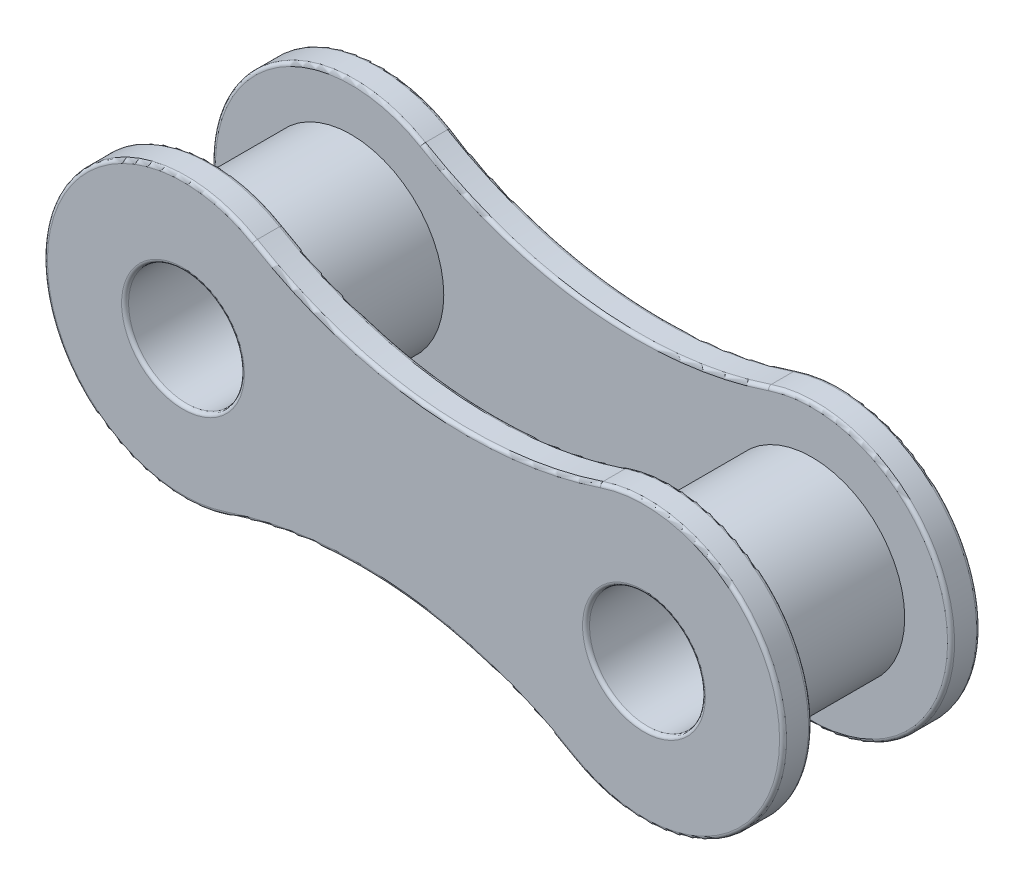
from build123d import *

# Parameters (mm, degrees)
BOSS_EXTRUDE1_DEPTH        = 3
BOSS_EXTRUDE1_DEPTH_BACK   = 3
SKETCH3_R                  = 4
SKETCH3_R_2                = 2.5
BOSS_EXTRUDE1_2_DEPTH      = 3
BOSS_EXTRUDE1_2_DEPTH_BACK = 3
SKETCH5_R                  = 2.5
BOSS_EXTRUDE2_DEPTH        = 1.25
FILLET1_R                  = 0.15
SCALE1_SCALE               = 0.5
SCALE2_SCALE               = 0.5
SCALE3_SCALE               = 0.5


with BuildPart() as part:
    # Sketch3 → Boss-Extrude1 (new, two sides: drawn at the far end of the back side and taken through both)
    with BuildSketch(Plane.XY.offset(-BOSS_EXTRUDE1_DEPTH_BACK)):
        with Locations((-87.399549733, 1.891684495)):
            Circle(SKETCH3_R)
        with Locations((-87.399549733, 1.891684495)):
            Circle(SKETCH3_R_2, mode=Mode.SUBTRACT)
    extrude(amount=BOSS_EXTRUDE1_DEPTH + BOSS_EXTRUDE1_DEPTH_BACK)


with BuildPart() as body_2:
    # Sketch3 → Boss-Extrude1 2 (new, two sides: drawn at the far end of the back side and taken through both)
    with BuildSketch(Plane.XY.offset(-BOSS_EXTRUDE1_2_DEPTH_BACK)):
        with Locations((-67.511724124, -0.223591499)):
            Circle(SKETCH3_R)
        with Locations((-67.511724124, -0.223591499)):
            Circle(SKETCH3_R_2, mode=Mode.SUBTRACT)
    extrude(amount=BOSS_EXTRUDE1_2_DEPTH + BOSS_EXTRUDE1_2_DEPTH_BACK)


with BuildPart() as body_3:
    # Sketch5 → Boss-Extrude2 (new body)
    with BuildSketch(Plane.XY.offset(3)):
        with BuildLine():
            ThreePointArc((-70.574575747, -5.382946104), (-61.545376441, -0.858174297), (-69.420828904, 5.464582104))
            ThreePointArc((-69.420828904, 5.464582104), (-77.051891637, 4.630059865), (-84.336698111, 7.0510391))
            ThreePointArc((-84.336698111, 7.0510391), (-93.365897416, 2.526267293), (-85.490444954, -3.796489108))
            ThreePointArc((-85.490444954, -3.796489108), (-77.85938222, -2.961966869), (-70.574575747, -5.382946104))
        make_face()
        with Locations((-67.511724124, -0.223591499)):
            Circle(SKETCH5_R, mode=Mode.SUBTRACT)
        with Locations((-87.399549733, 1.891684495)):
            Circle(SKETCH5_R, mode=Mode.SUBTRACT)
    extrude(amount=BOSS_EXTRUDE2_DEPTH)


with BuildPart() as body_4:
    # Mirror1: mirrored copy
    add(body_3.part.mirror(Plane.XY))


with BuildPart() as body_3_1:
    add(body_3.part)

    # Combine1: union part, body 4, body 2
    add(part.part)
    add(body_4.part)
    add(body_2.part)

    # Fillet1
    fillet1_edges = [body_3_1.edges().sort_by_distance(p)[0] for p in [
        (-70.011724124, -0.223591499, 4.25),
        (-77.051891637, 4.630059865, 4.25),
        (-89.899549733, 1.891684495, 4.25),
        (-93.365897416, 2.526267293, 4.25),
        (-70.011724124, -0.223591499, -4.25),
        (-89.899549733, 1.891684495, -4.25),
        (-77.85938222, -2.961966869, -3),
        (-61.545376441, -0.858174297, -3),
        (-77.051891637, 4.630059865, -3),
        (-93.365897416, 2.526267293, -3),
        (-77.85938222, -2.961966869, -4.25),
        (-61.545376441, -0.858174297, -4.25),
        (-77.051891637, 4.630059865, -4.25),
        (-93.365897416, 2.526267293, -4.25),
        (-77.85938222, -2.961966869, 4.25),
        (-93.365897416, 2.526267293, 3),
        (-77.051891637, 4.630059865, 3),
        (-61.545376441, -0.858174297, 3),
        (-77.85938222, -2.961966869, 3),
        (-61.545376441, -0.858174297, 4.25),
    ]]
    fillet(fillet1_edges, radius=FILLET1_R)


with BuildPart() as body_3_2:
    # Scale1: scaled about (-77.455636929, 0.834046498, 0)
    add(body_3_1.part.scale(SCALE1_SCALE).moved(Location((-38.727818464, 0.417023249, 0))))


with BuildPart() as body_3_3:
    # Scale2: scaled about (-77.455636929, 0.834046498, 0)
    add(body_3_2.part.scale(SCALE2_SCALE).moved(Location((-38.727818464, 0.417023249, 0))))


with BuildPart() as body_3_4:
    # Scale3: scaled about (-77.455636929, 0.834046498, 0)
    add(body_3_3.part.scale(SCALE3_SCALE).moved(Location((-38.727818464, 0.417023249, 0))))


solid = body_3_4.part
